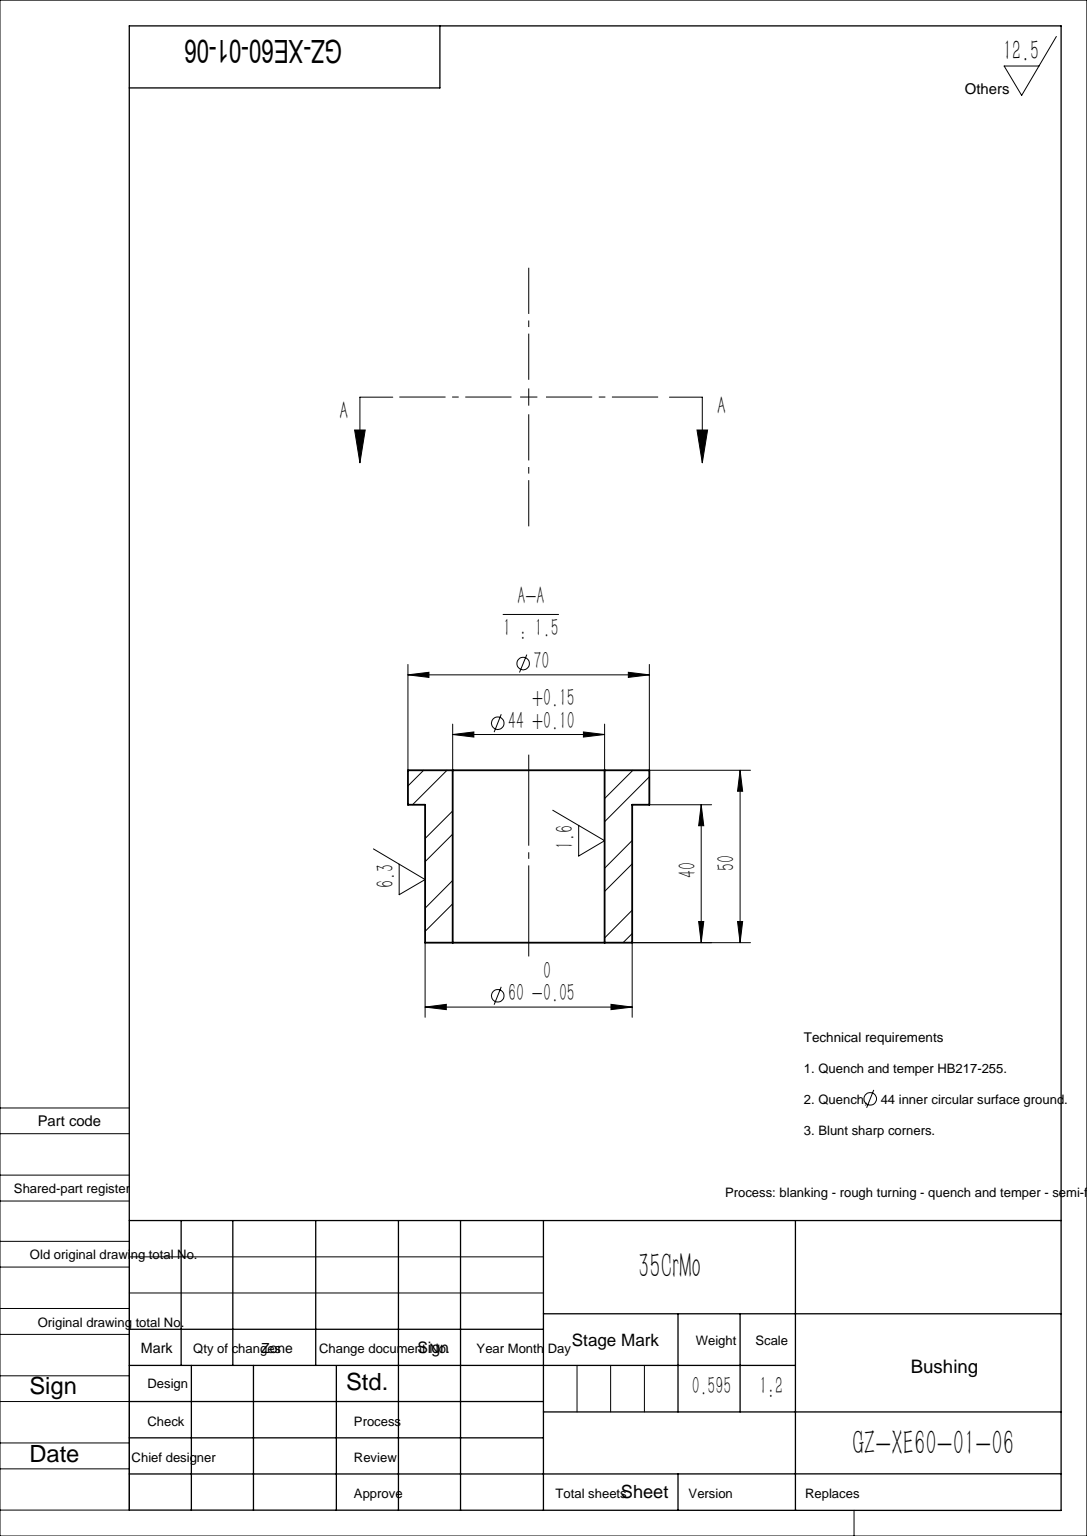
from build123d import *
from build123d.topology import SkipClean

# Parameters (mm, degrees)
SKETCH1_R           = 30
SKETCH1_R_2         = 22
BOSS_EXTRUDE1_DEPTH = 40
BOSS_EXTRUDE2_START = 10
SKETCH2_R           = 35
SKETCH2_R_2         = 22
BOSS_EXTRUDE2_DEPTH = 10


with BuildPart() as part:
    # Sketch1 → Boss-Extrude1 (new body)
    with BuildSketch(Plane.XY):
        Circle(SKETCH1_R)
        Circle(SKETCH1_R_2, mode=Mode.SUBTRACT)
    extrude(amount=BOSS_EXTRUDE1_DEPTH)

    # Sketch2 → Boss-Extrude2 (add)
    with SkipClean():  # the faces are left unmerged after this step: merging them gives an invalid solid
        with BuildSketch(Plane(origin=(0, 0, 0), x_dir=(-1, 0, 0), z_dir=(0, 0, -1)).offset(BOSS_EXTRUDE2_START)):
            Circle(SKETCH2_R)
            Circle(SKETCH2_R_2, mode=Mode.SUBTRACT)
        extrude(amount=-BOSS_EXTRUDE2_DEPTH)


solid = part.part
